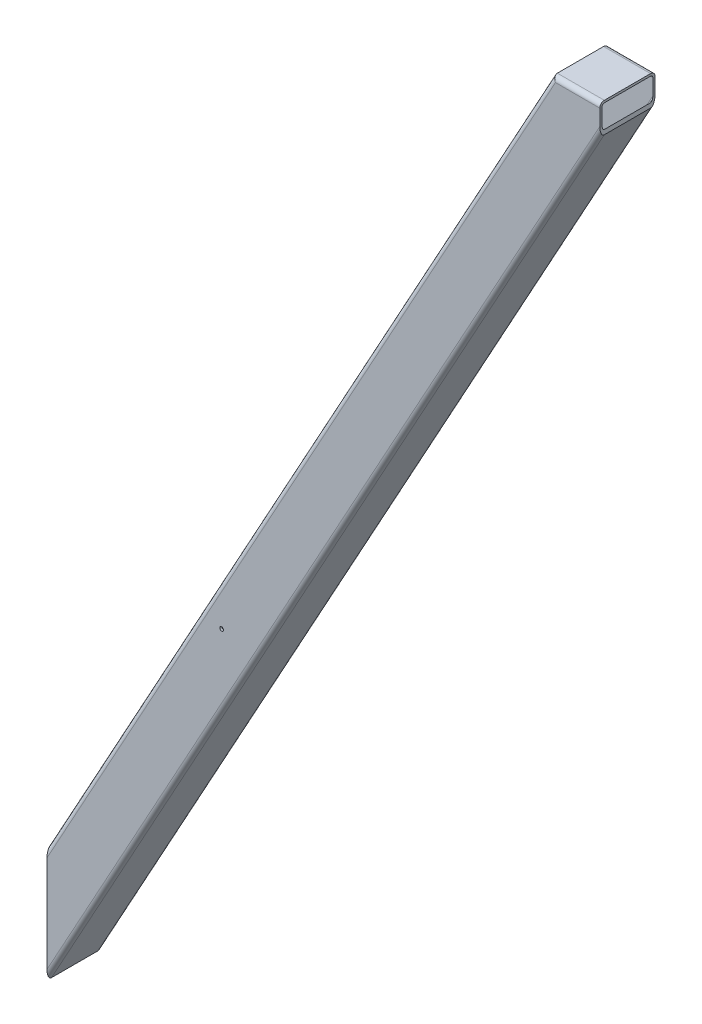
SolidWorks part; units mm, degrees
material "1023 碳钢板 (SS)"
ref_plane "Front Plane" through (0, 0, 0) normal (0, 0, 1) x (1, 0, 0)
ref_plane "Top Plane" through (0, 0, 0) normal (0, 1, 0) x (1, 0, 0)
ref_plane "Right Plane" through (0, 0, 0) normal (1, 0, 0) x (0, 0, -1)
sketch "Sketch1" plane through (0, 0, 0) normal (0, 0, 1) x (1, 0, 0)
  line L0 (0, 0) -> (0, 208.7368)
  line L1 (0, 208.7368) -> (915, 1874.4333)
  line L2 (915, 1874.4333) -> (1000, 1874.4333)
  line L3 (1000, 1874.4333) -> (1000, 1820.4333)
  line L4 (1000, 1820.4333) -> (0, 0)
  dimension "D1" = 85
  dimension "D2" = 1000
  dimension "54" = 54
  dimension "D3" = 2124.5
extrude "Boss-Extrude1" add sketch "Sketch1" along normal blind 100 contours L4 L0 L1 L2 L3
shell "Shell1" thickness 4
fillet "Fillet1" radius 8.2 6 edges at (500, 910.2167, 0) (457.5, 1041.5851, 0) (957.5, 1874.4333, 0) (957.5, 1874.4333, 100) (500, 910.2167, 100) (457.5, 1041.5851, 100)
fillet "Fillet2" radius 4.2 6 edges at (958.6832, 1870.4333, 96) (958.6832, 1870.4333, 4) (500, 918.5247, 96) (500, 918.5247, 4) (458.6832, 1035.431, 4) (458.6832, 1035.431, 96)
sketch "Sketch2" plane through (0, 0, 100) normal (0, 0, 1) x (1, 0, 0)
  line L0 (0, 17.0315) -> (0, 191.7053) construction
  circle A0 centre (316, 708.43) radius 17.2591
  dimension "D1" = 316
  dimension "D2" = 708.43
hole_wizard "M8 Tapped Hole1" positions "Sketch3" profile "Sketch4" tap size "M8" standard "ISO"
sketch "Sketch3" plane through (0, 0, 100) normal (0, 0, 1) x (1, 0, 0)
  point P0 (316, 708.43)
sketch "Sketch4" plane through (316, 708.43, 100) normal (1, 0, 0) x (0, -1, 0)
  line L0 (0, 0) -> (0, 21.7929)
  line L1 (0, 21.7929) -> (3.4, 19.75)
  line L2 (3.4, 19.75) -> (3.4, 0)
  line L5 (3.4, 0) -> (0, 0)
  line L10 (0, 21.7929) -> (-3.4, 19.75) construction
  line L11 (0, -6.35) -> (0, 107.95) construction
  dimension "螺纹孔钻头直径" = 6.8
  dimension "螺纹孔钻头深度" = 19.75
  dimension "导头角度" = 118
cosmetic thread "Hole Thread Line 1" parameters "D1"=16, "D2"=8
